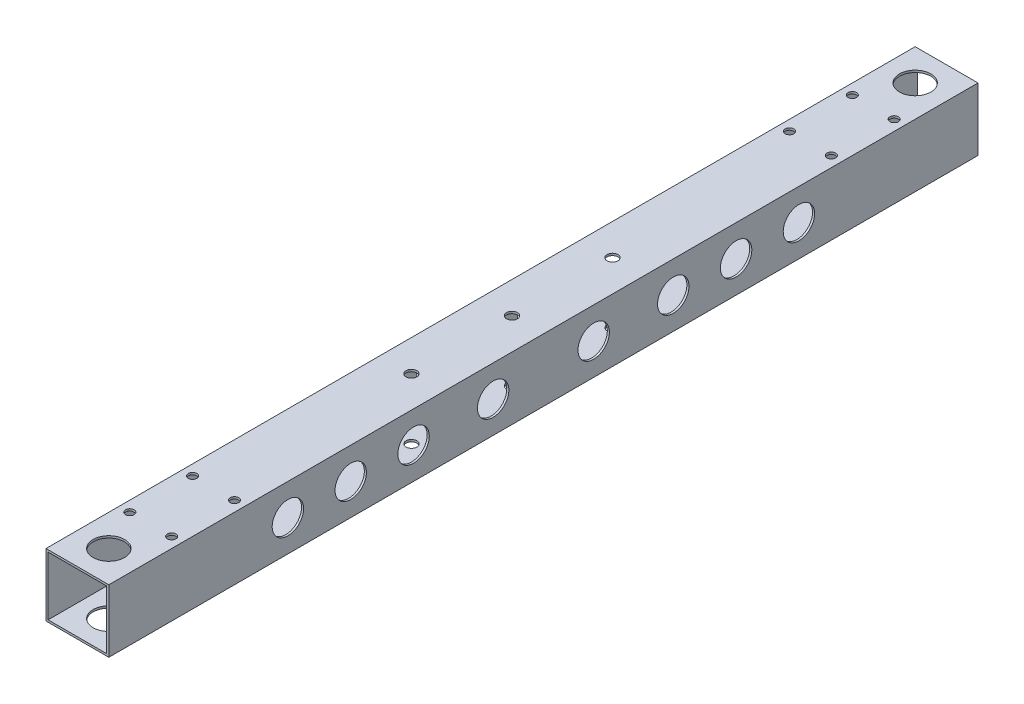
SolidWorks part; units mm, degrees
material "6061 合金"
ref_plane "前视基准面" through (0, 0, 0) normal (0, 0, 1) x (1, 0, 0)
ref_plane "上视基准面" through (0, 0, 0) normal (0, 1, 0) x (1, 0, 0)
ref_plane "右视基准面" through (0, 0, 0) normal (1, 0, 0) x (0, 0, -1)
other "Configuration Table"
sketch "草图1" plane through (0, 0, 0) normal (0, 0, 1) x (1, 0, 0)
  line L0 (-15, 15) -> (15, -15) construction
  line L1 (-15, -15) -> (15, -15)
  line L2 (-15, -15) -> (-15, 15)
  line L3 (-15, 15) -> (15, 15)
  line L4 (15, -15) -> (15, 15)
  point P4 (0, 0)
  dimension "D1" = 30
  dimension "D2" = 30
extrude "凸台-拉伸1" add sketch "草图1" along normal blind 415
shell "抽壳1" thickness 1
sketch "草图2" plane through (0, 15, 0) normal (0, 1, 0) x (1, 0, 0)
  line L0 (15, -415) -> (15, 0) construction
  line L1 (15, -415) -> (15, 0) construction
  line L2 (0, -159.5) -> (0, -255.5) construction
  line L3 (0, -207.5) -> (104.2949, -207.5) construction
  line L4 (-10, -350) -> (-10, -380) construction
  line L5 (-10, -65) -> (10, -65) construction
  line L6 (-10, -65) -> (-10, -35) construction
  line L7 (-10, -35) -> (10, -35) construction
  line L8 (10, -65) -> (10, -35) construction
  line L9 (-10, -350) -> (10, -350) construction
  line L10 (10, -350) -> (10, -380) construction
  line L11 (-10, -380) -> (10, -380) construction
  line L12 (15, 0) -> (-15, 0) construction
  circle A0 centre (0, -159.5) radius 2.6
  circle A1 centre (0, -255.5) radius 2.6
  circle A2 centre (0, -207.5) radius 2.6
  circle A3 centre (-10, -35) radius 2.05
  circle A4 centre (-10, -380) radius 2.05
  circle A5 centre (-10, -65) radius 2.05
  circle A6 centre (-10, -350) radius 2.05
  circle A7 centre (10, -65) radius 2.05
  circle A8 centre (10, -350) radius 2.05
  circle A9 centre (10, -35) radius 2.05
  circle A10 centre (10, -380) radius 2.05
  point P2 (0, -207.5)
  point P6 (15, -207.5)
  point P21 (0, -35)
  dimension "D2" = 5.2
  dimension "D3" = 35
  dimension "D6" = 4.1
  dimension "D1" = 96
  dimension "D4" = 20
  dimension "D5" = 30
extrude "切除-拉伸1" cut sketch "草图2" against normal through all
sketch "草图3" plane through (-15, 0, 0) normal (-1, 0, 0) x (0, 0, 1)
  line L0 (207.5, 15) -> (207.5, -15) construction
  line L1 (415, 15) -> (0, 15) construction
  line L2 (415, -15) -> (0, -15) construction
  line L3 (0, 15) -> (0, -15) construction
  circle A0 centre (85.5, 0) radius 7.5
  circle A1 centre (115.5, 0) radius 7.5
  circle A2 centre (145.5, 0) radius 7.5
  circle A3 centre (269.5, 0) radius 7.5
  circle A4 centre (299.5, 0) radius 7.5
  circle A5 centre (329.5, 0) radius 7.5
  circle A6 centre (183.5, 0) radius 7.5
  circle A7 centre (231.5, 0) radius 7.5
  point P11 (0, 0)
  point P26 (0, 0)
  dimension "D1" = 15
  dimension "D2" = 30
  dimension "D5" = 48
  dimension "D3" = 30
  dimension "D4" = 62
extrude "切除-拉伸2" cut sketch "草图3" against normal through all
sketch "草图4" plane through (0, 15, 0) normal (0, 1, 0) x (1, 0, 0)
  line L0 (-15, -207.5) -> (15, -207.5) construction
  line L1 (-15, -415) -> (-15, 0) construction
  line L2 (15, -415) -> (15, 0) construction
  line L3 (15, 0) -> (-15, 0) construction
  circle A0 centre (0, -15) radius 7.5
  circle A1 centre (0, -400) radius 7.5
  point P12 (0, 0)
  dimension "D1" = 15
  dimension "D2" = 15
extrude "切除-拉伸3" cut sketch "草图4" against normal through all
